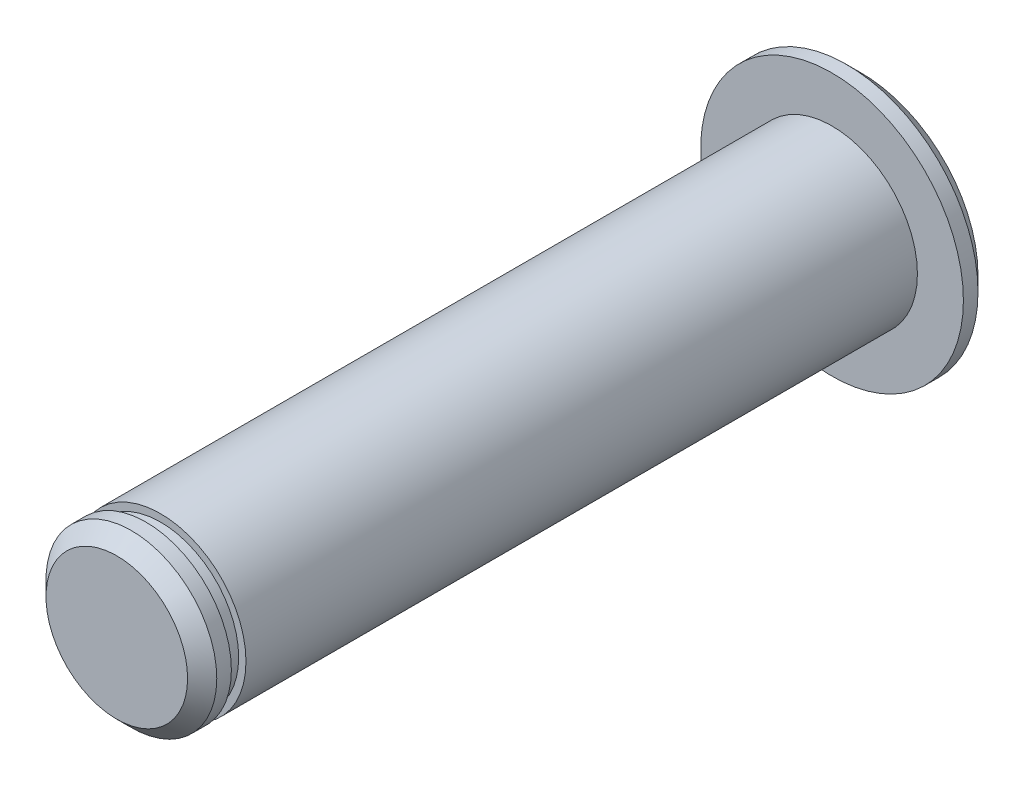
from build123d import *

# Parameters (mm, degrees)
SKETCH1_R           = 9
BOSS_EXTRUDE1_DEPTH = 2
SKETCH2_R           = 5.85
BOSS_EXTRUDE2_DEPTH = 46
SKETCH4_R           = 5.35
BOSS_EXTRUDE3_DEPTH = 1
SKETCH5_R           = 5.85
BOSS_EXTRUDE4_DEPTH = 2
CHAMFER1_SIZE       = 1


with BuildPart() as part:
    # Sketch1 → Boss-Extrude1 (new body)
    with BuildSketch(Plane.XY):
        Circle(SKETCH1_R)
    extrude(amount=BOSS_EXTRUDE1_DEPTH)

    # Sketch2 → Boss-Extrude2 (add)
    with BuildSketch(Plane.XY.offset(2)):
        Circle(SKETCH2_R)
    extrude(amount=BOSS_EXTRUDE2_DEPTH)

    # Sketch4 → Boss-Extrude3 (add)
    with BuildSketch(Plane.XY.offset(48)):
        Circle(SKETCH4_R)
    extrude(amount=BOSS_EXTRUDE3_DEPTH)

    # Sketch5 → Boss-Extrude4 (add)
    with BuildSketch(Plane.XY.offset(49)):
        Circle(SKETCH5_R)
    extrude(amount=BOSS_EXTRUDE4_DEPTH)

    # Chamfer1
    chamfer1_edges = [part.edges().sort_by_distance(p)[0] for p in [
        (-5.85, 0, 51),
        (-9, 0, 0),
    ]]
    chamfer(chamfer1_edges, length=CHAMFER1_SIZE)


solid = part.part
